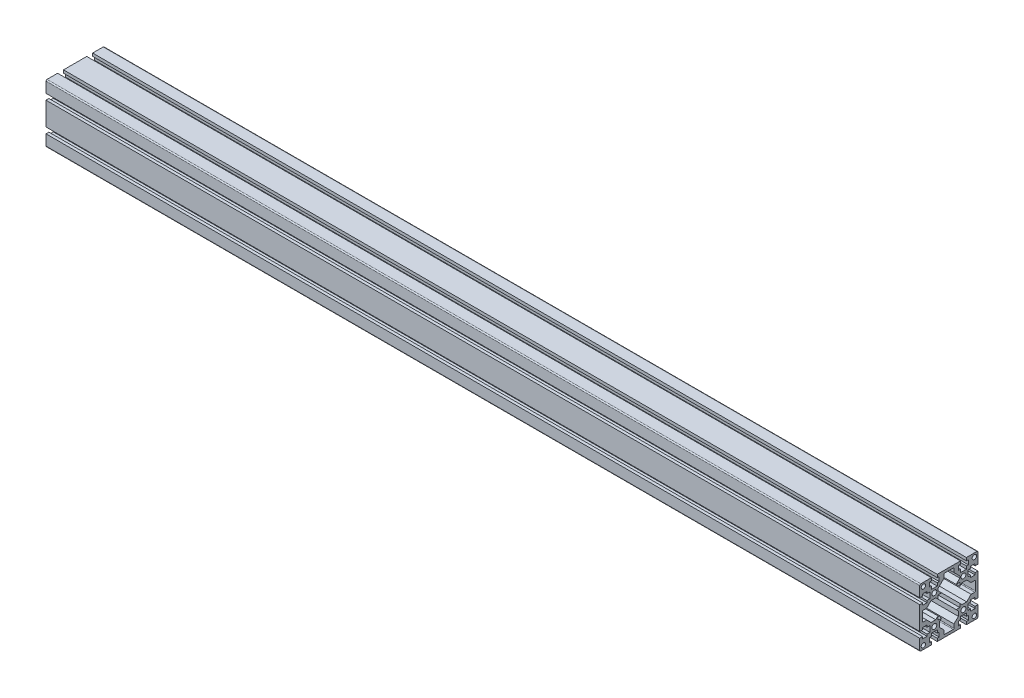
from build123d import *

# Parameters (mm, degrees)
SKETCH1_R                                = 3.4
SKETCH1_R_2                              = 3
ALUMINUM_PROFILE_80_X_80G_X_R1_5_1_DEPTH = 1200
SKETCH10_R                               = 3
CUT_EXTRUDE1_DEPTH                       = 1202.332593414


with BuildPart() as part:
    # Sketch1 → Aluminum profile 80 X 80G X R1.5(1) (new body)
    with BuildSketch(Plane.YZ.offset(-530.344827586)):
        with BuildLine():
            Line((-24.05, 40), (-24.05, 36))
            Line((-24.05, 36), (-26.75, 36))
            Line((-26.75, 36), (-26.75, 30))
            Line((-26.75, 30), (-24.05, 30))
            Line((-24.05, 30), (-24.05, 26))
            Line((-24.05, 26), (-15.95, 26))
            Line((-15.95, 26), (-15.95, 30))
            Line((-15.95, 30), (-13.25, 30))
            Line((-13.25, 30), (-13.25, 36))
            Line((-13.25, 36), (-15.95, 36))
            Line((-15.95, 36), (-15.95, 40))
            Line((-15.95, 40), (15.95, 40))
            Line((15.95, 40), (15.95, 36))
            Line((15.95, 36), (13.25, 36))
            Line((13.25, 36), (13.25, 30))
            Line((13.25, 30), (15.95, 30))
            Line((15.95, 30), (15.95, 26))
            Line((15.95, 26), (24.05, 26))
            Line((24.05, 26), (24.05, 30))
            Line((24.05, 30), (26.75, 30))
            Line((26.75, 30), (26.75, 36))
            Line((26.75, 36), (24.05, 36))
            Line((24.05, 36), (24.05, 40))
            Line((24.05, 40), (38.5, 40))
            ThreePointArc((38.5, 40), (39.560660172, 39.560660172), (40, 38.5))
            Line((40, 38.5), (40, 24.05))
            Line((40, 24.05), (36, 24.05))
            Line((36, 24.05), (36, 26.75))
            Line((36, 26.75), (30, 26.75))
            Line((30, 26.75), (30, 24.05))
            Line((30, 24.05), (26, 24.05))
            Line((26, 24.05), (26, 15.95))
            Line((26, 15.95), (30, 15.95))
            Line((30, 15.95), (30, 13.25))
            Line((30, 13.25), (36, 13.25))
            Line((36, 13.25), (36, 15.95))
            Line((36, 15.95), (40, 15.95))
            Line((40, 15.95), (40, -15.95))
            Line((40, -15.95), (36, -15.95))
            Line((36, -15.95), (36, -13.25))
            Line((36, -13.25), (30, -13.25))
            Line((30, -13.25), (30, -15.95))
            Line((30, -15.95), (26, -15.95))
            Line((26, -15.95), (26, -24.05))
            Line((26, -24.05), (30, -24.05))
            Line((30, -24.05), (30, -26.75))
            Line((30, -26.75), (36, -26.75))
            Line((36, -26.75), (36, -24.05))
            Line((36, -24.05), (40, -24.05))
            Line((40, -24.05), (40, -38.5))
            ThreePointArc((40, -38.5), (39.560660172, -39.560660172), (38.5, -40))
            Line((38.5, -40), (24.05, -40))
            Line((24.05, -40), (24.05, -36))
            Line((24.05, -36), (26.75, -36))
            Line((26.75, -36), (26.75, -30))
            Line((26.75, -30), (24.05, -30))
            Line((24.05, -30), (24.05, -26))
            Line((24.05, -26), (15.95, -26))
            Line((15.95, -26), (15.95, -30))
            Line((15.95, -30), (13.25, -30))
            Line((13.25, -30), (13.25, -36))
            Line((13.25, -36), (15.95, -36))
            Line((15.95, -36), (15.95, -40))
            Line((15.95, -40), (-15.95, -40))
            Line((-15.95, -40), (-15.95, -36))
            Line((-15.95, -36), (-13.25, -36))
            Line((-13.25, -36), (-13.25, -30))
            Line((-13.25, -30), (-15.95, -30))
            Line((-15.95, -30), (-15.95, -26))
            Line((-15.95, -26), (-24.05, -26))
            Line((-24.05, -26), (-24.05, -30))
            Line((-24.05, -30), (-26.75, -30))
            Line((-26.75, -30), (-26.75, -36))
            Line((-26.75, -36), (-24.05, -36))
            Line((-24.05, -36), (-24.05, -40))
            Line((-24.05, -40), (-38.5, -40))
            ThreePointArc((-38.5, -40), (-39.560660172, -39.560660172), (-40, -38.5))
            Line((-40, -38.5), (-40, -24.05))
            Line((-40, -24.05), (-36, -24.05))
            Line((-36, -24.05), (-36, -26.75))
            Line((-36, -26.75), (-30, -26.75))
            Line((-30, -26.75), (-30, -24.05))
            Line((-30, -24.05), (-26, -24.05))
            Line((-26, -24.05), (-26, -15.95))
            Line((-26, -15.95), (-30, -15.95))
            Line((-30, -15.95), (-30, -13.25))
            Line((-30, -13.25), (-36, -13.25))
            Line((-36, -13.25), (-36, -15.95))
            Line((-36, -15.95), (-40, -15.95))
            Line((-40, -15.95), (-40, 15.95))
            Line((-40, 15.95), (-36, 15.95))
            Line((-36, 15.95), (-36, 13.25))
            Line((-36, 13.25), (-30, 13.25))
            Line((-30, 13.25), (-30, 15.95))
            Line((-30, 15.95), (-26, 15.95))
            Line((-26, 15.95), (-26, 24.05))
            Line((-26, 24.05), (-30, 24.05))
            Line((-30, 24.05), (-30, 26.75))
            Line((-30, 26.75), (-36, 26.75))
            Line((-36, 26.75), (-36, 24.05))
            Line((-36, 24.05), (-40, 24.05))
            Line((-40, 24.05), (-40, 38.5))
            ThreePointArc((-40, 38.5), (-39.560660172, 39.560660172), (-38.5, 40))
            Line((-38.5, 40), (-24.05, 40))
        make_face()
        with Locations((-20, 20)):
            Circle(SKETCH1_R, mode=Mode.SUBTRACT)
        with Locations((20, 20)):
            Circle(SKETCH1_R, mode=Mode.SUBTRACT)
        with Locations((20, -20)):
            Circle(SKETCH1_R, mode=Mode.SUBTRACT)
        with Locations((-20, -20)):
            Circle(SKETCH1_R, mode=Mode.SUBTRACT)
        with Locations((-35, 35)):
            Circle(SKETCH1_R_2, mode=Mode.SUBTRACT)
        with Locations((35, 35)):
            Circle(SKETCH1_R_2, mode=Mode.SUBTRACT)
        with Locations((35, -35)):
            Circle(SKETCH1_R_2, mode=Mode.SUBTRACT)
        with BuildLine():
            Line((-13, 18), (-10, 15))
            Line((-10, 15), (-15, 15))
            Line((-15, 15), (-15, 10))
            Line((-15, 10), (-18, 13))
            Line((-18, 13), (-24.5, 13))
            Line((-24.5, 13), (-30.5, 7))
            Line((-30.5, 7), (-35.5, 7))
            ThreePointArc((-35.5, 7), (-36.207106781, 6.707106781), (-36.5, 6))
            Line((-36.5, 6), (-36.5, -6))
            ThreePointArc((-36.5, -6), (-36.207106781, -6.707106781), (-35.5, -7))
            Line((-35.5, -7), (-30.5, -7))
            Line((-30.5, -7), (-24.5, -13))
            Line((-24.5, -13), (-18, -13))
            Line((-18, -13), (-15, -10))
            Line((-15, -10), (-15, -15))
            Line((-15, -15), (-10, -15))
            Line((-10, -15), (-13, -18))
            Line((-13, -18), (-13, -24.5))
            Line((-13, -24.5), (-7, -30.5))
            Line((-7, -30.5), (-7, -35.5))
            ThreePointArc((-7, -35.5), (-6.707106781, -36.207106781), (-6, -36.5))
            Line((-6, -36.5), (6, -36.5))
            ThreePointArc((6, -36.5), (6.707106781, -36.207106781), (7, -35.5))
            Line((7, -35.5), (7, -30.5))
            Line((7, -30.5), (13, -24.5))
            Line((13, -24.5), (13, -18))
            Line((13, -18), (10, -15))
            Line((10, -15), (15, -15))
            Line((15, -15), (15, -10))
            Line((15, -10), (20, -15))
            Line((20, -15), (22.5, -15))
            Line((22.5, -15), (30.5, -7))
            Line((30.5, -7), (35.5, -7))
            ThreePointArc((35.5, -7), (36.207106781, -6.707106781), (36.5, -6))
            Line((36.5, -6), (36.5, 6))
            ThreePointArc((36.5, 6), (36.207106781, 6.707106781), (35.5, 7))
            Line((35.5, 7), (30.5, 7))
            Line((30.5, 7), (22.5, 15))
            Line((22.5, 15), (20, 15))
            Line((20, 15), (15, 10))
            Line((15, 10), (15, 15))
            Line((15, 15), (10, 15))
            Line((10, 15), (13, 18))
            Line((13, 18), (13, 24.5))
            Line((13, 24.5), (7, 30.5))
            Line((7, 30.5), (7, 35.5))
            ThreePointArc((7, 35.5), (6.707106781, 36.207106781), (6, 36.5))
            Line((6, 36.5), (-6, 36.5))
            ThreePointArc((-6, 36.5), (-6.707106781, 36.207106781), (-7, 35.5))
            Line((-7, 35.5), (-7, 30.5))
            Line((-7, 30.5), (-13, 24.5))
            Line((-13, 24.5), (-13, 18))
        make_face(mode=Mode.SUBTRACT)
    extrude(amount=ALUMINUM_PROFILE_80_X_80G_X_R1_5_1_DEPTH)

    # Sketch10 → Cut-Extrude1 (cut, through all)
    with BuildSketch(Plane(origin=(669.655172414, 0, 0), x_dir=(0, 0, -1), z_dir=(1, 0, 0))):
        with Locations((35, -35)):
            Circle(SKETCH10_R)
    extrude(amount=-CUT_EXTRUDE1_DEPTH, mode=Mode.SUBTRACT)


solid = part.part
